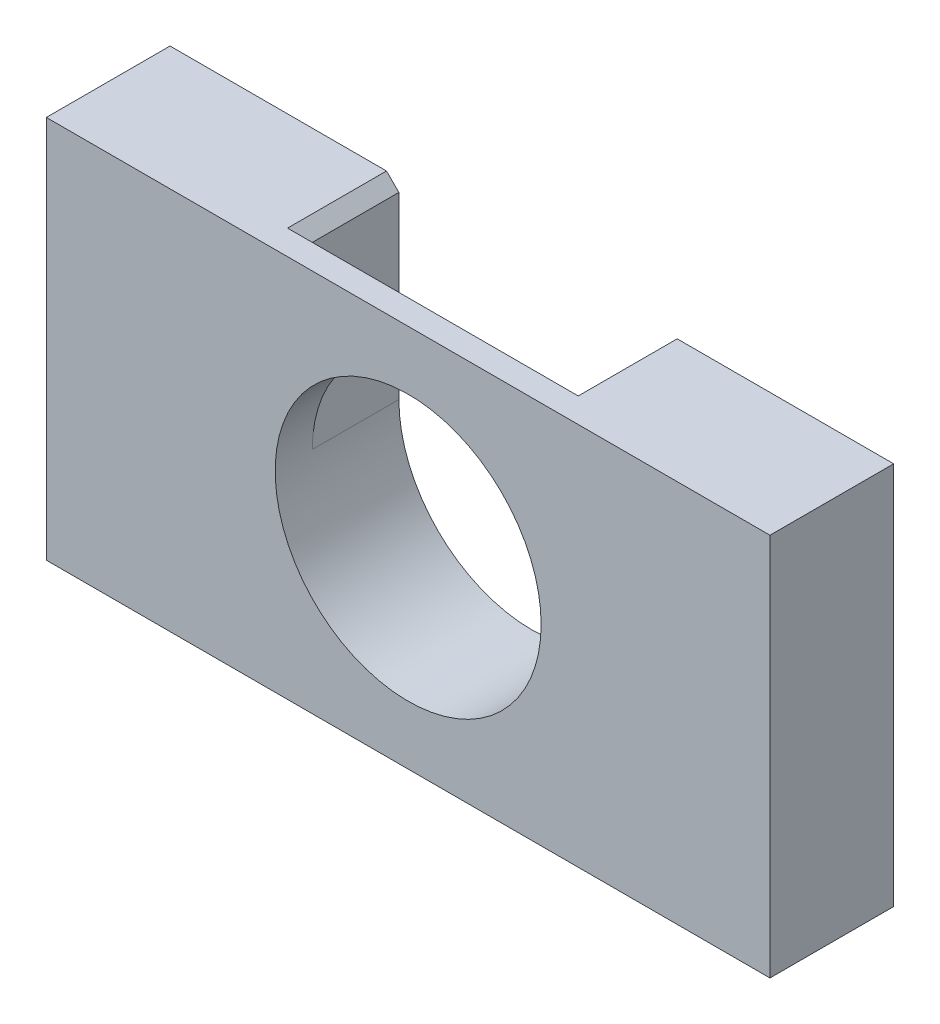
from build123d import *

# Parameters (mm, degrees)
SKETCH_1_W          = 117
SKETCH_1_H          = 62
EXTRUDE_1_DEPTH     = 20
CUT_EXTRUDE_1_REACH = 71.161
SKETCH_2_R          = 21.5
SKETCH_3_W          = 43
SKETCH_3_H          = 31
CUT_EXTRUDE_2_DEPTH = 14
CHAMFER_1_SIZE      = 2


with BuildPart() as part:
    # 草图1 → 凸台-拉伸1 (new body)
    with BuildSketch(Plane.XY):
        Rectangle(SKETCH_1_W, SKETCH_1_H)
    extrude(amount=EXTRUDE_1_DEPTH)

    # 草图2 → 切除-拉伸1 (cut, up to next)
    with BuildSketch(Plane.XY.offset(20), mode=Mode.PRIVATE) as cut_extrude_1_sk1:
        Circle(SKETCH_2_R)
    cut_extrude_1_tool1 = extrude(cut_extrude_1_sk1.sketch, amount=-CUT_EXTRUDE_1_REACH, mode=Mode.PRIVATE) & part.part
    add(cut_extrude_1_tool1.solids().sort_by_distance((0, 0, 20))[0], mode=Mode.SUBTRACT)

    # 草图3 → 切除-拉伸2 (cut)
    with BuildSketch(Plane(origin=(0, 0, 0), x_dir=(-1, 0, 0), z_dir=(0, 0, -1))):
        with Locations((0, 15.5)):
            Rectangle(SKETCH_3_W, SKETCH_3_H)
    extrude(amount=-CUT_EXTRUDE_2_DEPTH, mode=Mode.SUBTRACT)

    # 倒角1
    chamfer_1_edges = [part.edges().sort_by_distance(p)[0] for p in [
        (0, 31, 14),
        (21.5, 31, 7),
        (-21.5, 31, 7),
    ]]
    chamfer(chamfer_1_edges, length=CHAMFER_1_SIZE)


solid = part.part
